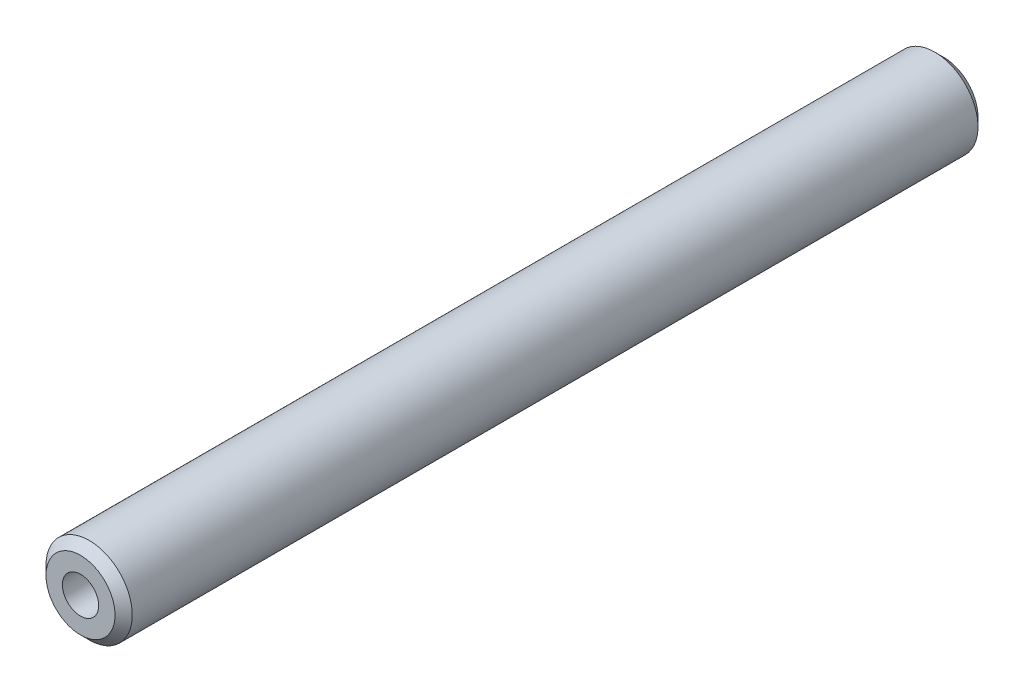
SolidWorks part; units mm, degrees
ref_plane "前视基准面" through (0, 0, 0) normal (0, 0, 1) x (1, 0, 0)
ref_plane "上视基准面" through (0, 0, 0) normal (0, 1, 0) x (1, 0, 0)
ref_plane "右视基准面" through (0, 0, 0) normal (1, 0, 0) x (0, 0, -1)
ref_plane "基准面4" through (0, 0, 0) normal (0, -1, 0) x (1, 0, 0)
sketch "草图1" plane through (0, 0, 0) normal (0, -1, 0) x (1, 0, 0)
  line L0 (2.1, 37.6) -> (0, 36.3382)
  line L1 (0, 36.3382) -> (0, -36.3382)
  line L2 (0, -36.3382) -> (2.1, -37.6)
  line L3 (2.1, -37.6) -> (2.1, -50)
  line L4 (2.1, -50) -> (4, -50)
  line L5 (4, -50) -> (5, -49)
  line L6 (5, -49) -> (5, 49)
  line L7 (5, 49) -> (4, 50)
  line L8 (4, 50) -> (2.1, 50)
  line L9 (2.1, 50) -> (2.1, 37.6)
  line L10 (0, 50) -> (0, -50) construction
revolve "旋转1" add sketch "草图1" angle 360 about L10
